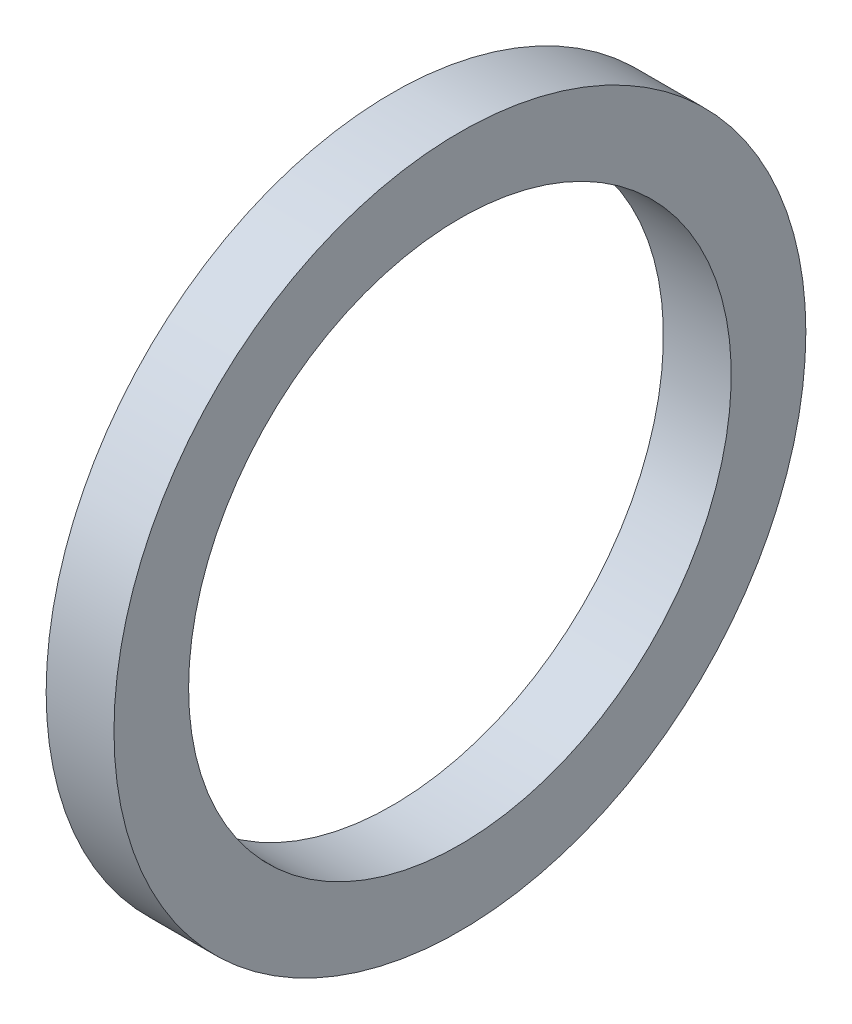
SolidWorks part; units mm, degrees
material "ASTM A36 钢"
ref_plane "前视基准面" through (0, 0, 0) normal (0, 0, 1) x (1, 0, 0)
ref_plane "上视基准面" through (0, 0, 0) normal (0, 1, 0) x (1, 0, 0)
ref_plane "右视基准面" through (0, 0, 0) normal (1, 0, 0) x (0, 0, -1)
other "Configuration Table"
sketch "草图1" plane through (0, 0, 0) normal (0, 1, 0) x (1, 0, 0)
  line L0 (-329.8236, 0) -> (16140.4427, 0) construction
  line L1 (0, 20) -> (5, 20)
  line L2 (0, 20) -> (0, 25.5)
  line L3 (0, 25.5) -> (5, 25.5)
  line L4 (5, 20) -> (5, 25.5)
  dimension "D1" = 40
  dimension "D2" = 51
  dimension "D3" = 5
revolve "旋转1" add sketch "草图1" angle 360 about L0
